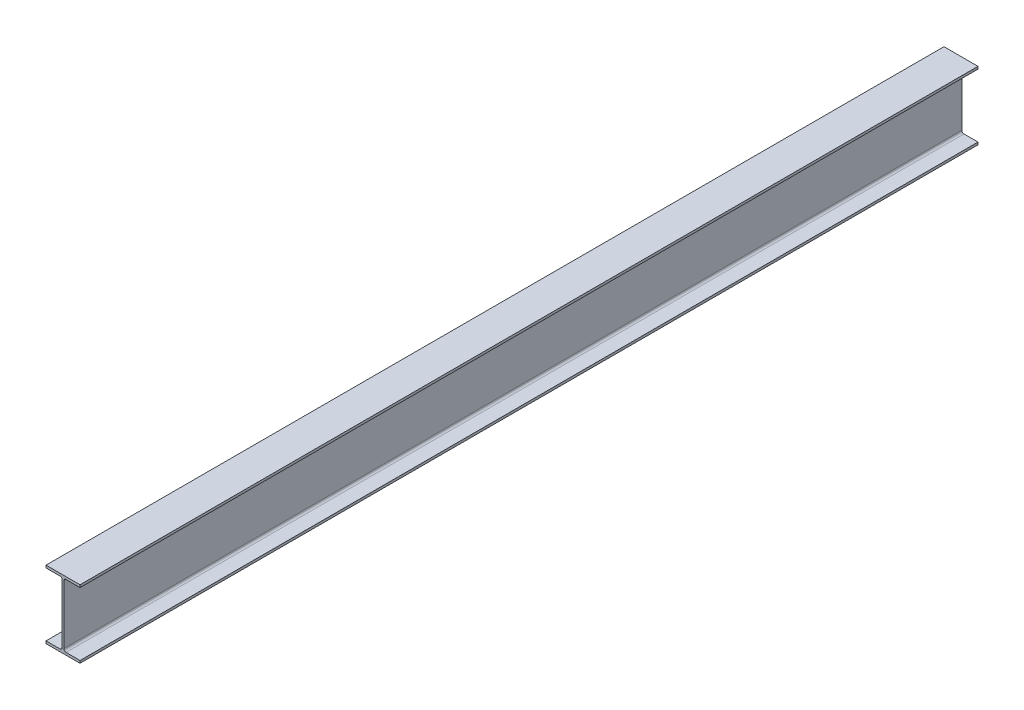
SolidWorks part; units mm, degrees
ref_plane "Front Plane" through (0, 0, 0) normal (0, 0, 1) x (1, 0, 0)
ref_plane "Top Plane" through (0, 0, 0) normal (0, 1, 0) x (1, 0, 0)
ref_plane "Right Plane" through (0, 0, 0) normal (1, 0, 0) x (0, 0, -1)
other "Configuration Table"
sketch "Sketch1" plane through (0, 0, 0) normal (0, 0, 1) x (1, 0, 0)
  line L0 (0, 0) -> (0, 250) construction
  line L1 (62.5, 0) -> (-62.5, 0)
  line L2 (-62.5, 0) -> (-62.5, 9)
  line L3 (-62.5, 9) -> (-11, 9)
  line L4 (3, 17) -> (3, 233)
  line L6 (-62.5, 241) -> (-62.5, 250)
  line L7 (-62.5, 250) -> (62.5, 250)
  line L8 (-3, 17) -> (-3, 233)
  line L9 (62.5, 241) -> (62.5, 250)
  line L10 (11, 241) -> (62.5, 241)
  line L11 (62.5, 9) -> (11, 9)
  line L12 (62.5, 0) -> (62.5, 9)
  line L13 (-11, 241) -> (-62.5, 241)
  arc A0 (11, 9) -> (3, 17) centre (11, 17) cw
  arc A1 (-3, 17) -> (-11, 9) centre (-11, 17) cw
  arc A2 (3, 233) -> (11, 241) centre (11, 233) cw
  arc A3 (-3, 233) -> (-11, 241) centre (-11, 233) ccw
  point P18 (3, 9)
  point P21 (-3, 9)
  point P24 (3, 241)
  point P27 (-3, 241)
  dimension "D6" = 8
  dimension "D1" = 250
  dimension "D2" = 125
  dimension "D3" = 6
  dimension "D4" = 9
  dimension "D5" = 9
extrude "Boss-Extrude1" add sketch "Sketch1" along normal blind 3300
